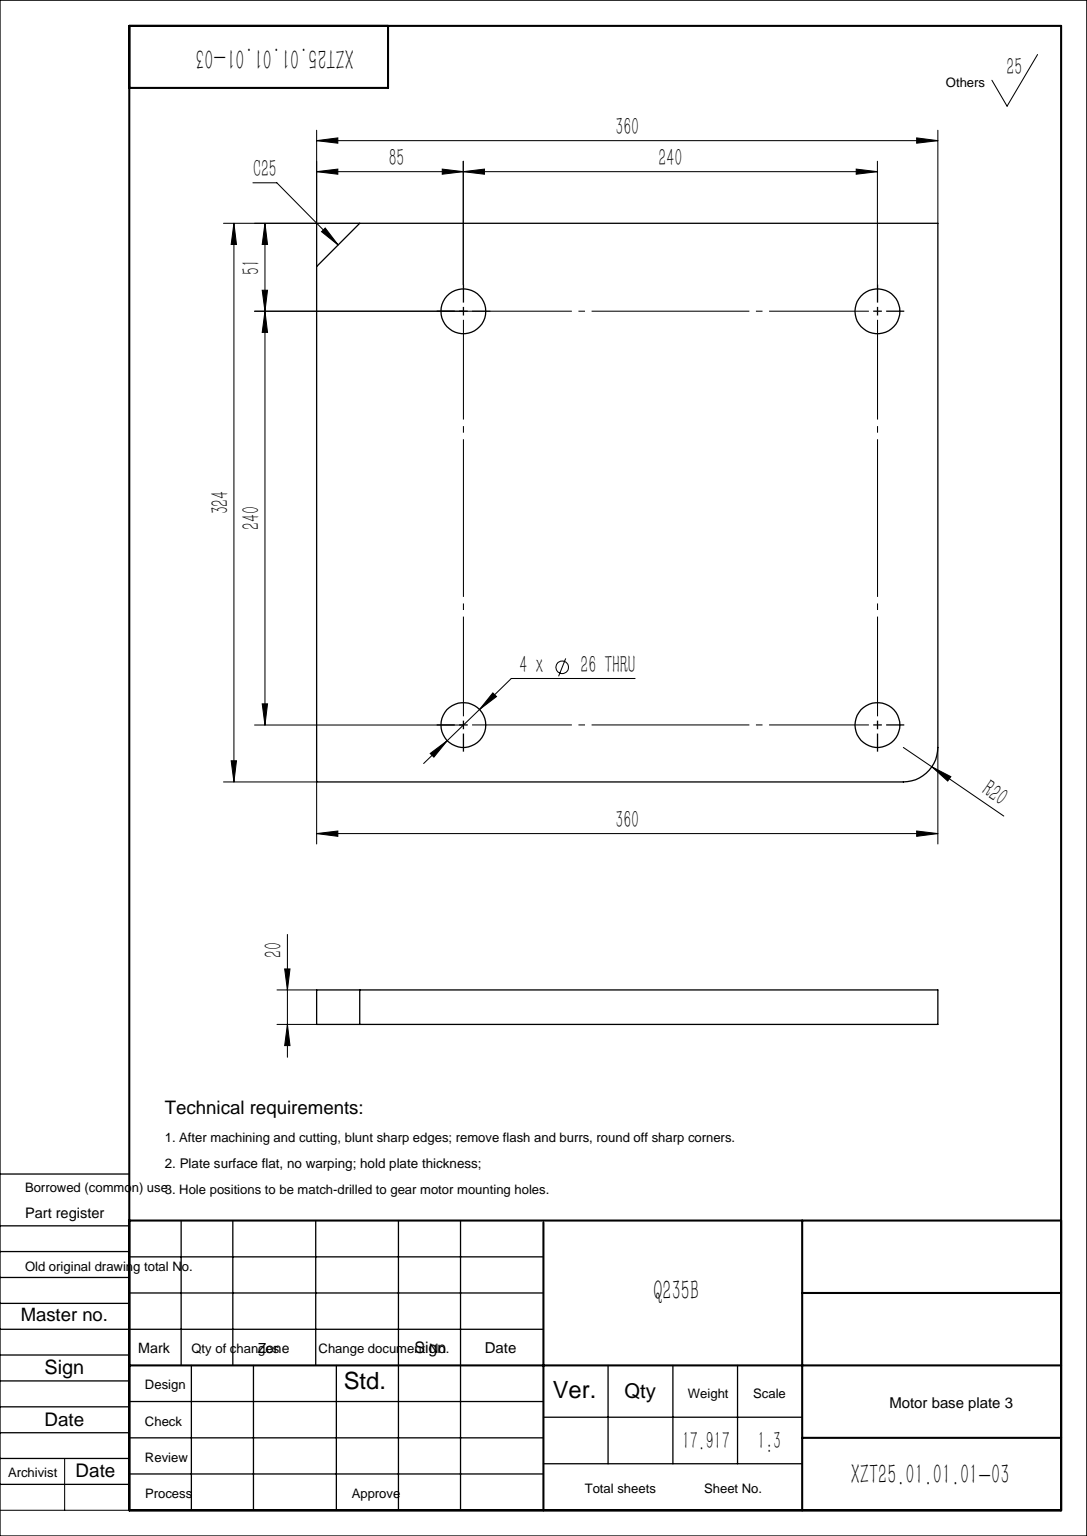
from build123d import *

# Parameters (mm, degrees)
SKETCH1_W                  = 360
SKETCH1_H                  = 324
BOSS_EXTRUDE1_DEPTH        = 10
CHAMFER1_SIZE              = 25
FILLET1_R                  = 20
F_25_0_25_DIAMETER_HOLE1_D = 26


with BuildPart() as part:
    # Sketch1 → Boss-Extrude1 (new, symmetric)
    with BuildSketch(Plane.XY):
        with Locations((180, 162)):
            Rectangle(SKETCH1_W, SKETCH1_H)
    extrude(amount=BOSS_EXTRUDE1_DEPTH, both=True)

    # Chamfer1
    chamfer1_edges = [part.edges().sort_by_distance(p)[0] for p in [
        (0, 324, 0),
    ]]
    chamfer(chamfer1_edges, length=CHAMFER1_SIZE)

    # Fillet1
    fillet1_edges = [part.edges().sort_by_distance(p)[0] for p in [
        (360, 0, 0),
    ]]
    fillet(fillet1_edges, radius=FILLET1_R)

    # Ø25.0 (25) Diameter Hole1 (through all)
    with Locations(Plane.XY.offset(10)):
        with Locations((85, 33), (325, 33), (325, 273), (85, 273)):
            Hole(F_25_0_25_DIAMETER_HOLE1_D / 2)


solid = part.part
